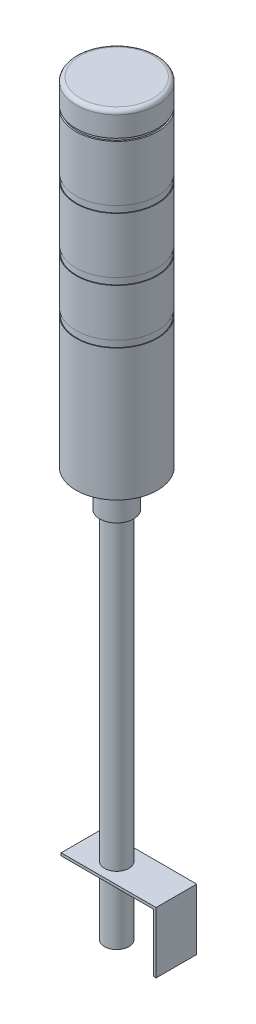
from build123d import *

# Parameters (mm, degrees)
SKETCH_2_R           = 24
SHELL_1_T            = -5
SKETCH_4_R           = 60
EXTRUDE_1_DEPTH      = 6
SKETCH_5_W           = 200
SKETCH_5_H           = 250
EXTRUDE_2_DEPTH      = 280
SKETCH_6_R           = 30
EXTRUDE_3_DEPTH      = 97.1
SKETCH_7_R           = 29.5
EXTRUDE_4_DEPTH      = 5
SKETCH_8_R           = 30
EXTRUDE_5_DEPTH      = 35
SKETCH_9_R           = 29.5
EXTRUDE_6_DEPTH      = 5
SKETCH_10_R          = 30
EXTRUDE_7_DEPTH      = 41
SKETCH_11_R          = 29.5
EXTRUDE_8_DEPTH      = 5
SKETCH_12_R          = 30
EXTRUDE_9_DEPTH      = 41
SKETCH_13_R          = 29
EXTRUDE_10_DEPTH     = 2
SKETCH_14_R          = 30
EXTRUDE_11_DEPTH     = 18
FILLET_1_R           = 3
SKETCH_15_OUTSIDE_W  = 599.076
SKETCH_15_OUTSIDE_H  = 512.576
SKETCH_15_OUTSIDE_R  = 22.5
CUT_EXTRUDE_1_DEPTH  = 26
SKETCH_16_W          = 1000.950512006
SKETCH_16_H          = 1372.546192884
CUT_EXTRUDE_12_DEPTH = 1285.766986682
SKETCH_17_R          = 12.5
EXTRUDE_13_DEPTH     = 27
SKETCH_24_R          = 9
EXTRUDE_1_2_DEPTH    = 275
EXTRUDE_1_3_DEPTH    = 15


with BuildPart() as part:
    # 扫描4: sweep along a path in 草图1
    with BuildLine(Plane.XY) as sweep_4_path:
        Line((0, 0), (0, 202.5))
        ThreePointArc((0, 202.5), (8.786796564, 223.713203436), (30, 232.5))
        Line((30, 232.5), (182.5, 232.5))
        ThreePointArc((182.5, 232.5), (203.713203436, 241.286796564), (212.5, 262.5))
        Line((212.5, 262.5), (212.5, 698.5))
    # 草图2 → 扫描4 (sweep)
    with BuildSketch(Plane(origin=(0, 0, 0), x_dir=(1, 0, 0), z_dir=(0, 1, 0))):
        Circle(SKETCH_2_R)
    sweep(path=sweep_4_path.line)

    # 抽壳1
    shell_1_openings = [part.faces().sort_by_distance(p)[0] for p in [
        (0, 0, 0),
    ]]
    offset(amount=SHELL_1_T, openings=shell_1_openings, kind=Kind.INTERSECTION)

    # 草图4 → Extrude 1 (add)
    with BuildSketch(Plane(origin=(0, 698.5, 0), x_dir=(-1, 0, 0), z_dir=(0, 1, 0))):
        with Locations(Location((-212.5, 0, 0), (0, 0, 90))):
            Circle(SKETCH_4_R)
    extrude(amount=EXTRUDE_1_DEPTH)

    # 草图5 → 拉伸2 (add)
    with BuildSketch(Plane(origin=(0, 704.5, 0), x_dir=(-1, 0, 0), z_dir=(0, 1, 0))):
        with Locations((-212.5, 0)):
            Rectangle(SKETCH_5_W, SKETCH_5_H)
    extrude(amount=EXTRUDE_2_DEPTH)

    # 草图6 → 拉伸3 (add)
    with BuildSketch(Plane(origin=(0, 984.5, 0), x_dir=(-1, 0, 0), z_dir=(0, 1, 0))):
        with Locations(Location((-212.5, -75, 0), (0, 0, 270))):
            Circle(SKETCH_6_R)
    extrude(amount=EXTRUDE_3_DEPTH)

    # 草图7 → 拉伸4 (add)
    with BuildSketch(Plane(origin=(0, 1081.6, 0), x_dir=(-1, 0, 0), z_dir=(0, 1, 0))):
        with Locations(Location((-212.5, -75, 0), (0, 0, 90))):
            Circle(SKETCH_7_R)
    extrude(amount=EXTRUDE_4_DEPTH)

    # 草图8 → 拉伸5 (add)
    with BuildSketch(Plane(origin=(0, 1086.6, 0), x_dir=(-1, 0, 0), z_dir=(0, 1, 0))):
        with Locations(Location((-212.5, -75, 0), (0, 0, 270))):
            Circle(SKETCH_8_R)
    extrude(amount=EXTRUDE_5_DEPTH)

    # 草图9 → 拉伸6 (add)
    with BuildSketch(Plane(origin=(0, 1121.6, 0), x_dir=(-1, 0, 0), z_dir=(0, 1, 0))):
        with Locations(Location((-212.5, -75, 0), (0, 0, 90))):
            Circle(SKETCH_9_R)
    extrude(amount=EXTRUDE_6_DEPTH)

    # 草图10 → 拉伸7 (add)
    with BuildSketch(Plane(origin=(0, 1126.6, 0), x_dir=(-1, 0, 0), z_dir=(0, 1, 0))):
        with Locations(Location((-212.5, -75, 0), (0, 0, 270))):
            Circle(SKETCH_10_R)
    extrude(amount=EXTRUDE_7_DEPTH)

    # 草图11 → 拉伸8 (add)
    with BuildSketch(Plane(origin=(0, 1167.6, 0), x_dir=(-1, 0, 0), z_dir=(0, 1, 0))):
        with Locations(Location((-212.5, -75, 0), (0, 0, 90))):
            Circle(SKETCH_11_R)
    extrude(amount=EXTRUDE_8_DEPTH)

    # 草图12 → 拉伸9 (add)
    with BuildSketch(Plane(origin=(0, 1172.6, 0), x_dir=(-1, 0, 0), z_dir=(0, 1, 0))):
        with Locations(Location((-212.5, -75, 0), (0, 0, 270))):
            Circle(SKETCH_12_R)
    extrude(amount=EXTRUDE_9_DEPTH)

    # 草图13 → 拉伸10 (add)
    with BuildSketch(Plane(origin=(0, 1213.6, 0), x_dir=(-1, 0, 0), z_dir=(0, 1, 0))):
        with Locations(Location((-212.5, -75, 0), (0, 0, 90))):
            Circle(SKETCH_13_R)
    extrude(amount=EXTRUDE_10_DEPTH)

    # 草图14 → 拉伸11 (add)
    with BuildSketch(Plane(origin=(0, 1215.6, 0), x_dir=(-1, 0, 0), z_dir=(0, 1, 0))):
        with Locations(Location((-212.5, -75, 0), (0, 0, 270))):
            Circle(SKETCH_14_R)
    extrude(amount=EXTRUDE_11_DEPTH)

    # 圆角1
    fillet_1_edges = [part.edges().sort_by_distance(p)[0] for p in [
        (212.5, 1233.6, -45),
    ]]
    fillet(fillet_1_edges, radius=FILLET_1_R)

    # 草图15 outside → 切除-拉伸1 (cut)
    with BuildSketch(Plane.XZ):
        with Locations((144.25, 0)):
            Rectangle(SKETCH_15_OUTSIDE_W, SKETCH_15_OUTSIDE_H)
        with Locations(Location((0, 0, 0), (0, 0, 270))):
            Circle(SKETCH_15_OUTSIDE_R, mode=Mode.SUBTRACT)
    extrude(amount=-CUT_EXTRUDE_1_DEPTH, mode=Mode.SUBTRACT)

    # 草图16 → 拉伸12 (cut, through all)
    with BuildSketch(Plane(origin=(312.5, 0, 0), x_dir=(0, 0, -1), z_dir=(1, 0, 0))):
        with Locations((-375.475256003, 298.226903558)):
            Rectangle(SKETCH_16_W, SKETCH_16_H)
    extrude(amount=-CUT_EXTRUDE_12_DEPTH, mode=Mode.SUBTRACT)

    # 草图17 → 拉伸13 (add)
    with BuildSketch(Plane.XZ.offset(-984.5)):
        with Locations(Location((212.5, -75, 0), (0, 0, 90))):
            Circle(SKETCH_17_R)
    extrude(amount=EXTRUDE_13_DEPTH)

    # 草图24 → Extrude 1 2 (add)
    with BuildSketch(Plane.XZ.offset(-957.5)):
        with Locations(Location((212.5, -75, 0), (0, 0, 270))):
            Circle(SKETCH_24_R)
    extrude(amount=EXTRUDE_1_2_DEPTH)

    # 草图26 → Extrude 1 3 (add, symmetric)
    with BuildSketch(Plane.XY.offset(-75)):
        Polygon((186.5, 732.5), (256.5, 732.5), (256.5, 687.5), (254.5, 687.5), (254.5, 730.5), (186.5, 730.5), align=None)
    extrude(amount=EXTRUDE_1_3_DEPTH, both=True)


solid = part.part
